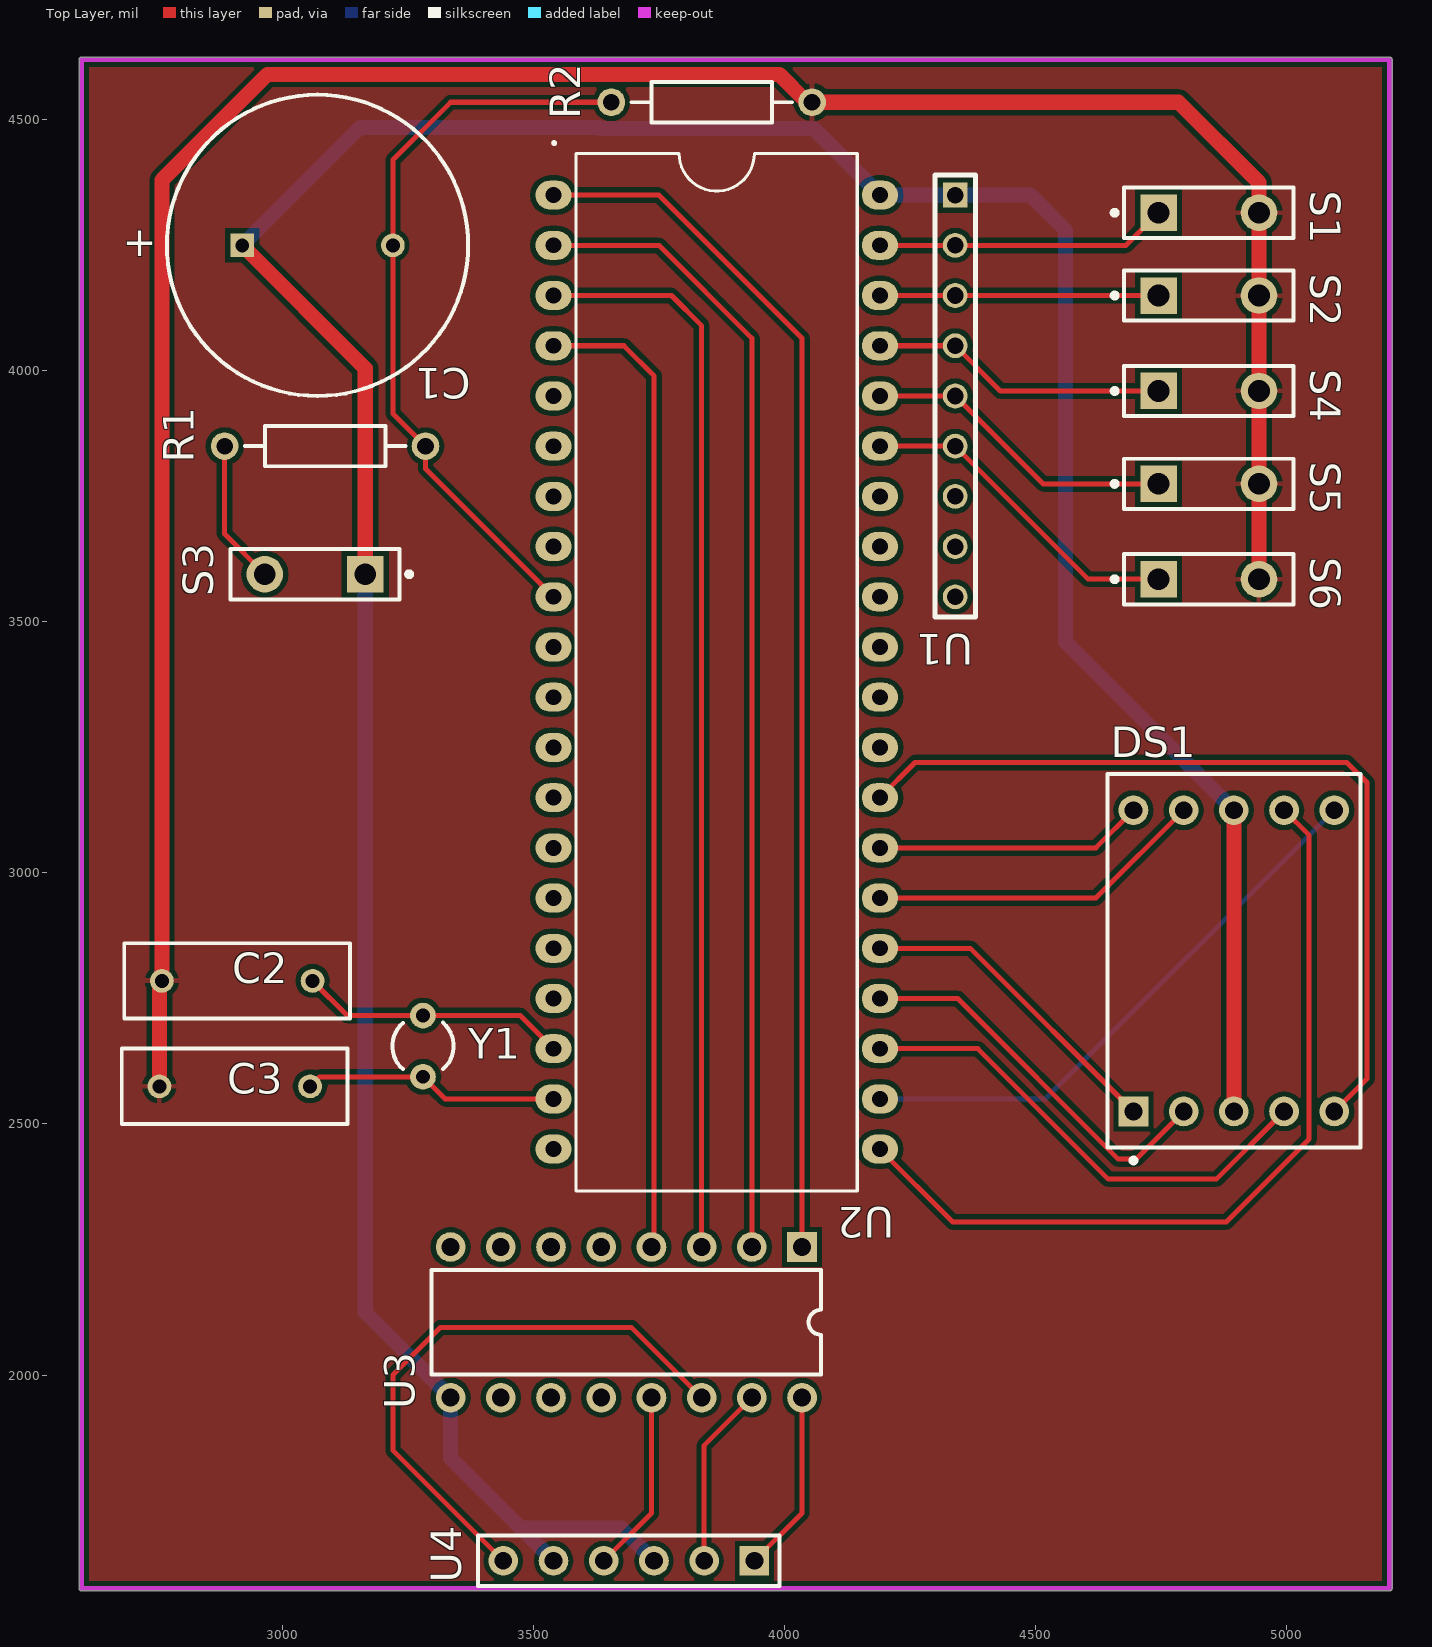
[diagram p0: Top Layer view]
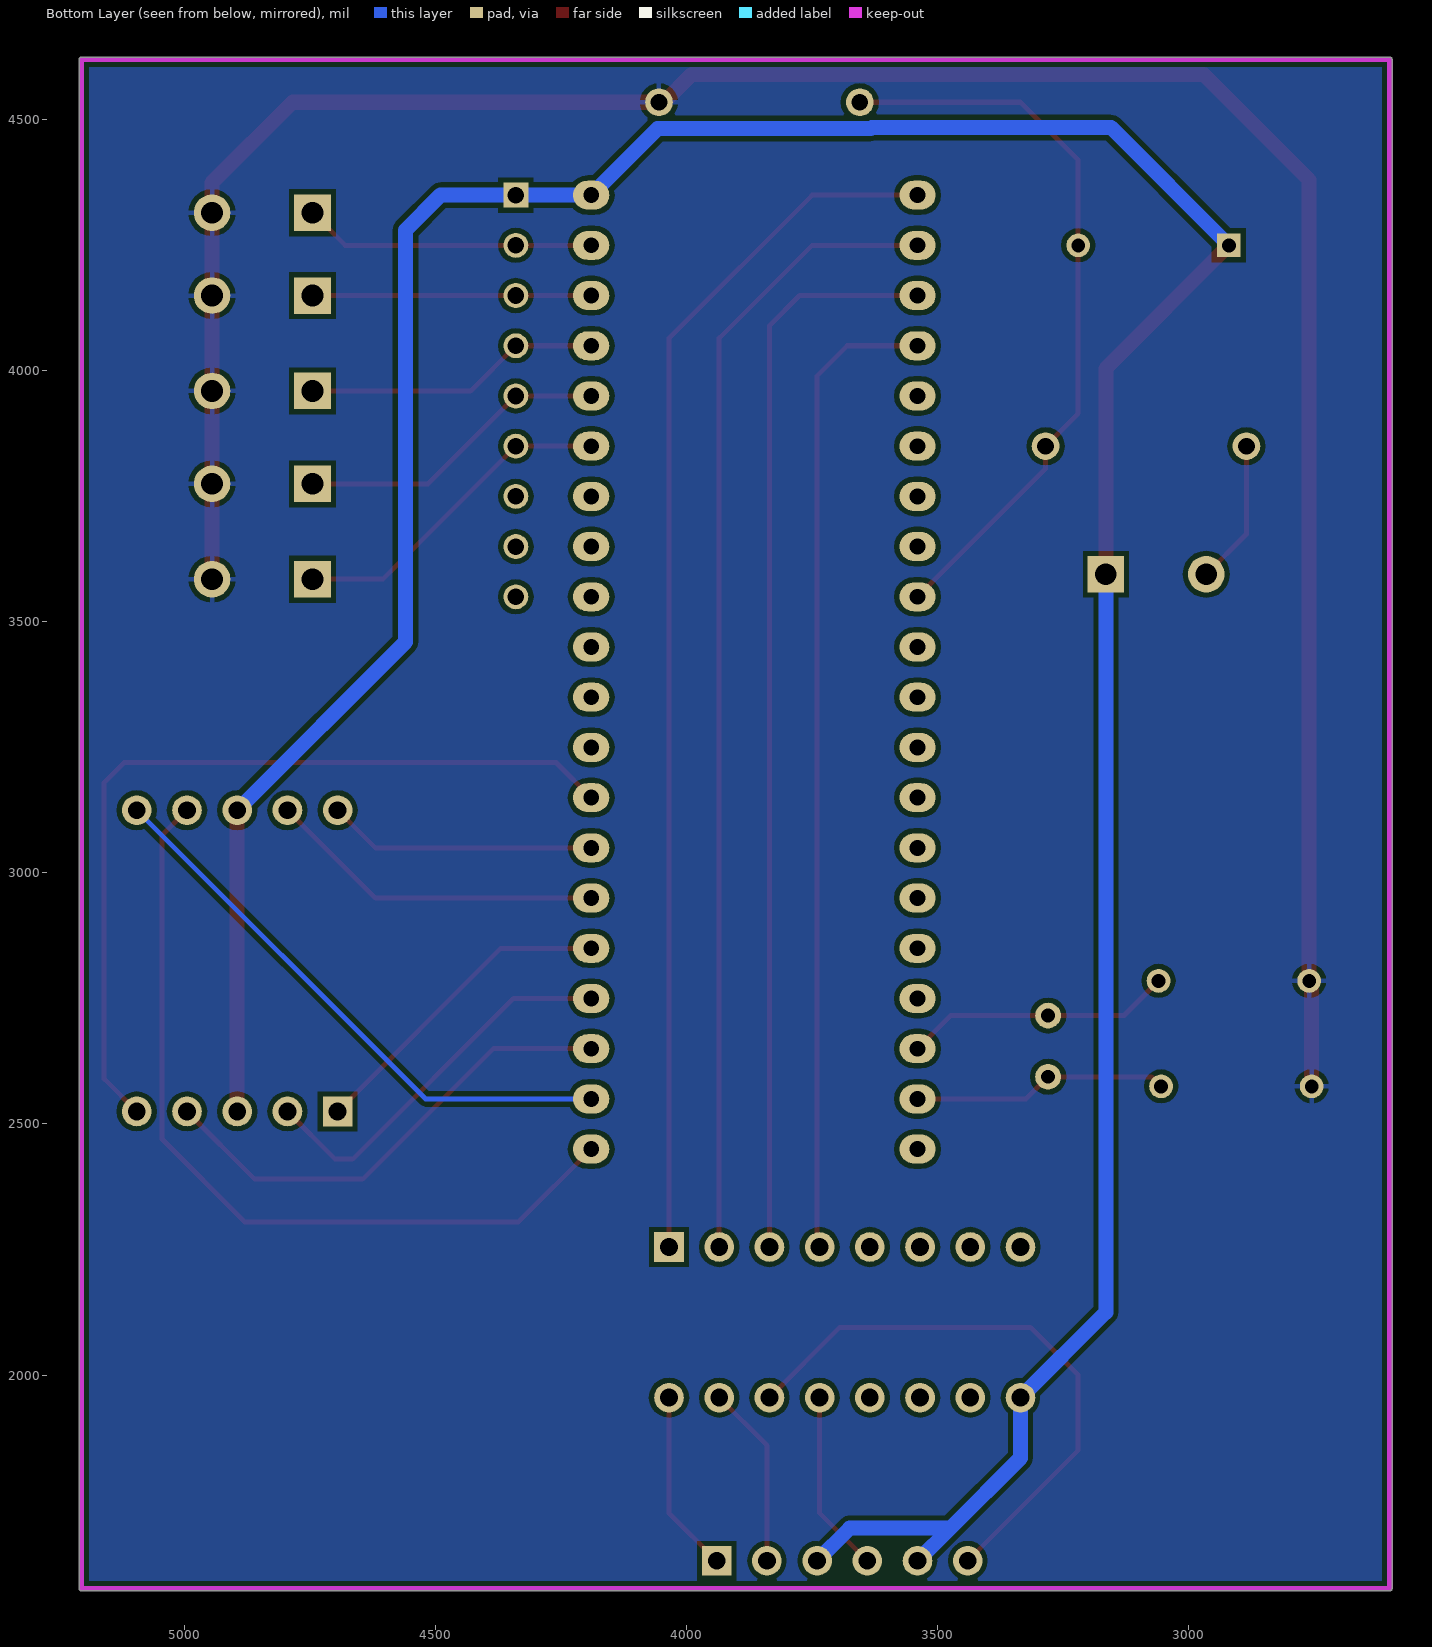
[diagram p1: Bottom Layer view, seen from below]
# Altium PCB MISC82904.PcbDoc
Units mil, origin at the board's own origin, x right, y up, seen from the top; angles counter-clockwise.
Board outline 2615.03 x 3055.03 mil, 2 copper layers (Top Layer, Bottom Layer); 17 components, 27 nets, 105 pads, 0 vias.

## Layer stack, top to bottom (the 12.6 mil dielectric is the usual default, probably not edited)
Top Solder: solder mask 0.4, Solder Resist, Dk 3.5
Top Layer: signal copper 1.4
Dielectric 1: dielectric 12.6, FR-4, Dk 4.8
Bottom Layer: signal copper 1.4
Bottom Solder: solder mask 0.4, Solder Resist, Dk 3.5

## Board outline
2594.99,1575 ccw(c2600,1575) 2600,1569.98 5205,1569.98 ccw(c5205,1575) 5210.02,1575 5210.02,4620 ccw(c5205,4620) 5205,4625.02 2600,4625.02 ccw(c2600,4620) 2594.99,4620

## Design rules (kind name [scope] priority, off if disabled: settings)
Clearance [All] p1: gap=10
MinimumSolderMaskSliver [All] p1: minsoldermaskwidth=0
PolygonConnect [All] p1: connectstyle=Relief reliefconductorwidth=10 reliefentries=4 polygonreliefangle="90 Angle" airgapwidth=10
RoutingVias [All] p1: holewidth=28 width=50 viastyle="Through Hole" minholewidth=28 minwidth=50 maxholewidth=28 maxwidth=50
SilkToSilkClearance [All] p1: silktosilkclearance=0
SilkToSolderMaskClearance [IsPad] p1: minsilkscreentomaskgap=0 clearancetoexposedcopper=TRUE
SolderMaskExpansion [All] p1: expansion=4
Width [All] p1: maxlimit=30 minlimit=10 preferedwidth=10
27 further rules are at their usual default settings.

## Components (designator, comment, footprint, x,y, rotation, side; value= is the part's Value field where it differs from the comment)
C1 "10UF" RB7.6-15 3070,4250 r180 top
C2 "22PF" RAD-0.3 2910,2785 r0 top
C3 "22PF" RAD-0.3 2905,2575 r0 top
DS1 "Dpy Blue-CC" H 4895,2825 r0 top
R1 "220" AXIAL-0.4 3085,3850 r180 top
R2 "10K" AXIAL-0.4 3855,4535 r180 top
S1 "SW-PB" SPST-2 4845,4315 r0 top
S2 "SW-PB" SPST-2 4845,4150 r0 top
S3 "SW-PB" SPST-2 3065,3595 r180 top
S4 "SW-PB" SPST-2 4845,3960 r0 top
S5 "SW-PB" SPST-2 4845,3775 r0 top
S6 "SW-PB" SPST-2 4845,3585 r0 top
U1 "Resistor network" paizu 4340,3950 r270 top
U2 "STC89C52RC" STC89C52RC 3865,3410.33 r270 top
U3 "ULN2003A" A16 3685,2105 r180 top
U4 "Motor" HDR1X6 3940,1630 r180 top
Y1 "XTAL" R38 3280,2655 r180 top

## Footprints (in the part's own frame and the unit in brackets; to place one, negate y for a bottom-side part, rotate by r counter-clockwise, add the part's x,y. Pads: shape width x height; smd on the part's side, far side on the other; paste and mask are expansions set on the pad)
A16 [mm] "DIP; 16 Leads; Row Spacing 7.62 mm; Pitch 2.54 mm"
  rect 1.5x1.5 hole 0.9: 1(-8.89,-3.81)
  round 1.5 hole 0.9: 2(-6.35,-3.81) 3(-3.81,-3.81) 4(-1.27,-3.81) 5(1.27,-3.81) 6(3.81,-3.81) 7(6.35,-3.81) 8(8.89,-3.81) 9(8.89,3.81) 10(6.35,3.81) 11(3.81,3.81) 12(1.27,3.81) 13(-1.27,3.81) 14(-3.81,3.81) 15(-6.35,3.81) 16(-8.89,3.81)
  silkscreen extent -9.85,-2.65 9.85,2.65
AXIAL-0.4 [mm] "Axial Device, Thru-Hole; 2 Leads; 0.4 in Pin Spacing"
  round 1.4 hole 0.85: 1(-5.08,0) 2(5.08,0)
  silkscreen extent -4.06,-1.02 4.06,1.02
H [mm] "LED, 7-Segment Display, 14.2 mm, RHD; 10 Leads; Row Space 15.24 mm; Pitch 2.54 mm"
  rect 1.5x1.5 hole 0.9: 1(-5.08,-7.62)
  round 1.5 hole 0.9: 2(-2.54,-7.62) 3(0,-7.62) 4(2.54,-7.62) 5(5.08,-7.62) 6(5.08,7.62) 7(2.54,7.62) 8(0,7.62) 9(-2.54,7.62) 10(-5.08,7.62)
  silkscreen extent -6.4,-10.22 6.4,9.45, body extent -6.4,-9.45 6.4,9.45, height 8.25
HDR1X6 [mm] "Connector; Header; 6 Position"
  rect 1.5x1.5 hole 0.9: 1(0,0)
  round 1.5 hole 0.9: 2(2.54,0) 3(5.08,0) 4(7.62,0) 5(10.16,0) 6(12.7,0)
  silkscreen extent -1.27,-1.27 13.97,1.27
paizu [mm]
  rect 1.26x1.26 hole 0.84 paste+0 mask+0.051: 1(-10.16,0)
  round 1.26 hole 0.84 paste+0 mask+0.051: 2(-7.62,0) 3(-5.08,0) 4(-2.54,0) 5(0,0) 6(2.54,0) 7(5.08,0) 8(7.62,0) 9(10.16,0)
  silkscreen extent -11.18,-1.02 11.18,1.02
R38 [mm] "Crystal, Thru-Hole; 2 Leads; Body 3.1 x 8.2 mm (Dia.xH)"
  round 1.3 hole 0.7: 1(0,1.55) 2(0,-1.55)
  silkscreen extent -1.55,-1.19 1.55,1.17
RAD-0.3 [mm] "Radial Cap, Thru-Hole; 2 Leads; 0.3 in Pin Spacing"
  round 1.2 hole 0.7: 1(-3.81,0) 2(3.81,0)
  silkscreen extent -5.71,-1.91 5.71,1.91
RB7.6-15 [mm] "Polarized Capacitor (Radial); 2 Leads"
  rect 1.2x1.2 hole 0.7: 1(3.81,0)
  round 1.2 hole 0.7: 2(-3.81,0)
  silkscreen extent -7.62,-7.62 7.62,7.62
SPST-2 [mm] "Switch; 2 Leads"
  rect 1.85x1.85 hole 1.1: 1(-2.54,0)
  round 1.85 hole 1.1: 2(2.54,0)
  silkscreen extent -4.89,-1.27 4.28,1.27
STC89C52RC [mm]
  oval 1.467x1.833 hole 0.8 paste+0 mask+0.051: 1(-23.868,-8.255) 2(-21.328,-8.255) 3(-18.788,-8.255) 4(-16.248,-8.255) 5(-13.708,-8.255) 6(-11.168,-8.255) 7(-8.628,-8.255) 8(-6.088,-8.255) 9(-3.548,-8.255) 10(-1.008,-8.255) 11(1.532,-8.255) 12(4.072,-8.255) 13(6.612,-8.255) 14(9.152,-8.255) 15(11.692,-8.255) 16(14.232,-8.255) 17(16.772,-8.255) 18(19.312,-8.255) 19(21.852,-8.255) 20(24.392,-8.255) 21(24.392,8.255) 22(21.852,8.255) 23(19.312,8.255) 24(16.772,8.255) 25(14.232,8.255) 26(11.692,8.255) 27(9.152,8.255) 28(6.612,8.255) 29(4.072,8.255) 30(1.532,8.255) 31(-1.008,8.255) 32(-3.548,8.255) 33(-6.088,8.255) 34(-8.628,8.255) 35(-11.168,8.255) 36(-13.708,8.255) 37(-16.248,8.255) 38(-18.788,8.255) 39(-21.328,8.255) 40(-23.868,8.255)
  silkscreen extent -26.58,-8.3 26.5,7.11

## Part data
C1: library part "Cap Pol1", "Polarized Capacitor (Radial)"
C2 C3: library part Cap, "Capacitor"
DS1: "14.2 mm General Purpose Blue 7-Segment Display: CC, RH DP, Gray Surface"
R1 R2: library part Res2, "Resistor"
S1 S2 S3 S4 S5 S6: "Switch"
U1: library part 排阻
U3: "High-Voltage, High-Current Darlington Array"
U4: library part 电机
Y1: "Crystal Oscillator"

## Nets (pads, with @x,y where several pads share a name; then routed paths per layer and width w, separated by ;. In a path a pad name is that pad's centre, name@x,y a point inside that pad or via, vN(x,y) a via of type N, cw(c..) or ccw(c..) an arc to the next point about the centre after c; other vN are vias at no path point)
GND: C2.1 C3.1 R2.1 S1.2 S2.2 S4.2 S5.2 S6.2 | length 4958.1
  Top Layer w30: C3.1 2755,2780 C2.1 2760,4380 2970,4590 3990,4590 4045,4535 R2.1 4785,4535 4945,4375 S1.2 S2.2 S4.2 S5.2 S6.2
NetC1_2: C1.2 R1.1 R2.2 U2.9 | length 1485.2
  Top Layer w10: U2.9 3285,3805 R1.1 3220,3915 C1.2 3220,4420 3335,4535 R2.2
NetC2_2: C2.2 U2.18 Y1.2 | length 535.9
  Top Layer w10: C2.2 3128.98,2716.02 Y1.2 3473.98,2716.02 U2.18
NetC3_2: C3.2 U2.19 Y1.1 | length 511.1
  Top Layer w10: C3.2 3073.98,2593.98 Y1.1 3323.97,2550 U2.19
NetDS1_1: DS1.1 U2.25 | length 639.6
  Top Layer w10: U2.25 4370,2850 DS1.1
NetDS1_2: DS1.2 U2.24 | length 776.9
  Top Layer w10: U2.24 4345,2750 4665,2430 4700,2430 DS1.2
NetDS1_4: DS1.4 U2.23 | length 968.6
  Top Layer w10: U2.23 4385,2650 4645,2390 4860,2390 DS1.4
NetDS1_5: DS1.5 U2.28 | length 1697.5
  Top Layer w10: U2.28 4260,3220 5120,3220 5160,3180 5160,2590 DS1.5
NetDS1_6: DS1.6 U2.22 | length 1143.2
  Bottom Layer w10: U2.22 4520,2550 DS1.6
NetDS1_7: DS1.7 U2.21 | length 1659.1
  Top Layer w10: U2.21 4335,2305 4880,2305 5045,2470 5045,3075 DS1.7
NetDS1_9: DS1.9 U2.26 | length 677.5
  Top Layer w10: U2.26 4620,2950 DS1.9
NetDS1_10: DS1.10 U2.27 | length 536.1
  Top Layer w10: U2.27 4620,3050 DS1.10
NetR1_2: R1.2 S3.2 | length 288.1
  Top Layer w10: R1.2 2885,3675 S3.2
NetS1_1: S1.1 U1.2 U2.39 | length 581.9
  Top Layer w10: U2.39 U1.2 4680,4250 S1.1
NetS2_1: S2.1 U1.3 U2.38 | length 555
  Top Layer w10: U2.38 U1.3 S2.1
NetS4_1: S4.1 U1.4 U2.37 | length 592.3
  Top Layer w10: U2.37 U1.4 4430,3960 S4.1
NetS5_1: S5.1 U1.5 U2.36 | length 627.5
  Top Layer w10: U2.36 U1.5 4515,3775 S5.1
NetS6_1: S6.1 U1.6 U2.35 | length 664.8
  Top Layer w10: U2.35 U1.6 4605,3585 S6.1
NetU2_1: U2.1 U3.1 | length 2423
  Top Layer w10: U2.1 3750,4350 4035,4065 U3.1
NetU2_2: U2.2 U3.2 | length 2281.6
  Top Layer w10: U2.2 3750,4250 3935,4065 U3.2
NetU2_3: U2.3 U3.3 | length 2154.9
  Top Layer w10: U2.3 3775,4150 3835,4090 U3.3
NetU2_4: U2.4 U3.4 | length 1961.9
  Top Layer w10: U2.4 3680,4050 3740,3990 3740,2260 U3.4
NetU3_13: U3.13 U4.4 | length 364.4
  Top Layer w10: U4.4 3735,1725 U3.13
NetU3_14: U3.14 U4.6 | length 1173.5
  Top Layer w10: U4.6 3220,1850 3220,2000 3315,2095 3695,2095 U3.14
NetU3_15: U3.15 U4.2 | length 364.4
  Top Layer w10: U4.2 3840,1860 U3.15
NetU3_16: U3.16 U4.1 | length 364.4
  Top Layer w10: U4.1 4035,1725 U3.16
VCC: C1.1 DS1.3 DS1.8 S3.1 U1.1 U2.40 U3.9 U4.3 U4.5 | length 6884.8
  Top Layer w30: C1.1 3165,4005 S3.1 ; DS1.3 DS1.8
  Bottom Layer w30: C1.1 3155,4485 3630.67,4485 3633.23,4482.44 4057.56,4482.44 U2.40 4490,4350 4560,4280 4560,3460 DS1.8 ; S3.1 3165,2125 U3.9 3335,1835 3475,1695 ; U4.5 3475,1695 ; U4.3 3675,1695 3475,1695
pads on no net: U1.7 U1.8 U1.9 U2.5 U2.6 U2.7 U2.8 U2.10 U2.11 U2.12 U2.13 U2.14 U2.15 U2.16 U2.17 U2.20 U2.29 U2.30 U2.31 U2.32 U2.33 U2.34 U3.5 U3.6 U3.7 U3.8 U3.10 U3.11 U3.12

## Polygon pours and split planes (outlines as drawn)
GND on Bottom Layer "Top Layer-No Net" (solid, remove dead copper, pour order 0): 2090,4815 5660,4815 5790,4945 5685,4840 5685,825 2605,825 2165,1265
GND on Top Layer "Top Layer-No Net" (solid, remove dead copper, pour order 2): 1855,4940 1960,5045 5930,5045 5930,1110 5990,1050 5670,1370 1355,1370

## Keep-outs
Keep-Out Layer:
  lines w10: 3955,1575 5205,1575 5205,4575 5205,4620 2600,4620 2600,1575 3965,1575